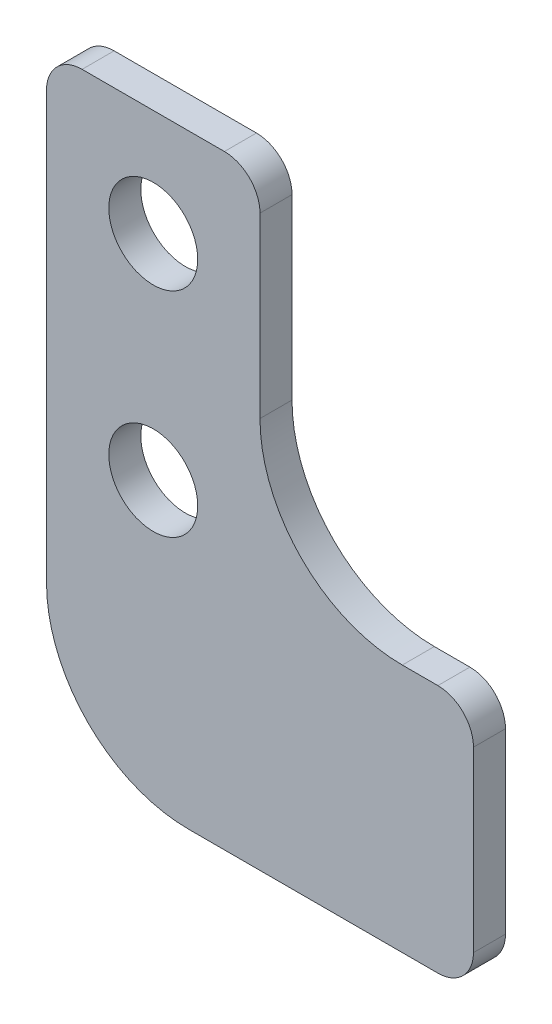
SolidWorks part; units mm, degrees
ref_plane "Front Plane" through (0, 0, 0) normal (0, 0, 1) x (1, 0, 0)
ref_plane "Top Plane" through (0, 0, 0) normal (0, 1, 0) x (1, 0, 0)
ref_plane "Right Plane" through (0, 0, 0) normal (1, 0, 0) x (0, 0, -1)
sketch "Sketch1" plane through (0, 0, 0) normal (0, 0, 1) x (1, 0, 0)
  line L0 (0, 85) -> (30, 85)
  line L1 (20, 0) -> (55, 0)
  line L2 (0, 20) -> (0, 80)
  line L3 (5, 85) -> (25, 85)
  line L4 (60, 5) -> (60, 30)
  line L5 (30, 80) -> (30, 55)
  line L7 (50, 35) -> (55, 35)
  circle A0 centre (15, 70) radius 6.25
  circle A1 centre (15, 40) radius 6.25
  arc A2 (30, 55) -> (50, 35) centre (50, 55) ccw
  arc A3 (55, 35) -> (60, 30) centre (55, 30) cw
  arc A4 (20, 0) -> (0, 20) centre (20, 20) cw
  arc A5 (0, 80) -> (5, 85) centre (5, 80) cw
  arc A6 (25, 85) -> (30, 80) centre (25, 80) cw
  arc A7 (55, 0) -> (60, 5) centre (55, 5) ccw
  point P15 (60, 35)
  point P18 (0, 0)
  point P27 (60, 0)
  dimension "D4" = 15
  dimension "D5" = 30
  dimension "D6" = 15
  dimension "D7" = 12.5
  dimension "D8" = 12.5
  dimension "D9" = 15
  dimension "D10" = 20
  dimension "D11" = 5
  dimension "D12" = 20
  dimension "D13" = 5
  dimension "D14" = 5
  dimension "D1" = 35
  dimension "D2" = 85
  dimension "D3" = 60
extrude "Boss-Extrude1" add sketch "Sketch1" along normal blind 4.5 contours L1 A7 L4 A3 L7 A2 L5 A6 L0 A5 L2 A4 A0 A1
